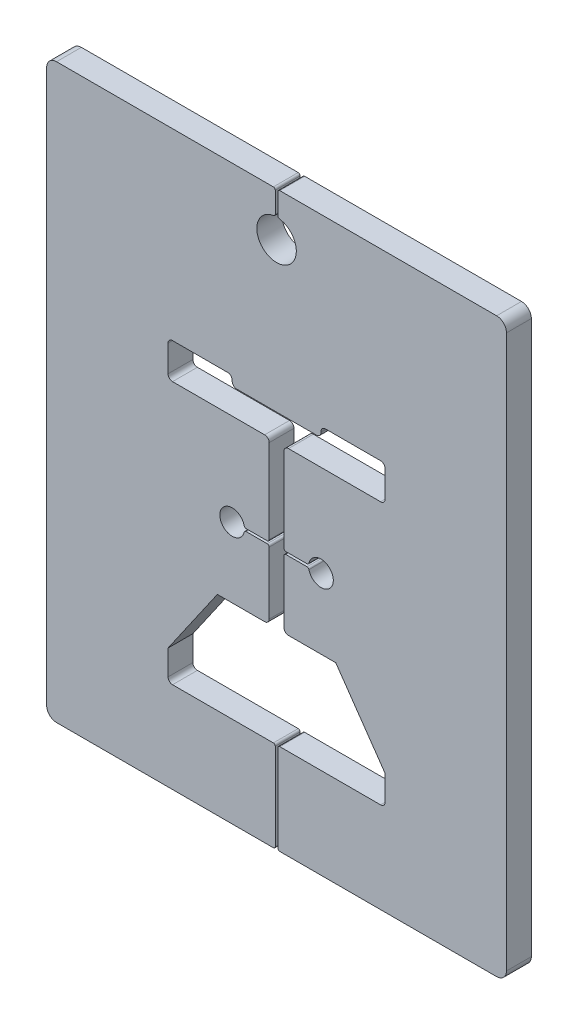
SolidWorks part; units mm, degrees
material "普通碳钢"
ref_plane "Front Plane" through (0, 0, 0) normal (0, 0, 1) x (1, 0, 0)
ref_plane "Top Plane" through (0, 0, 0) normal (0, 1, 0) x (1, 0, 0)
ref_plane "Right Plane" through (0, 0, 0) normal (1, 0, 0) x (0, 0, -1)
sketch "Sketch1" plane through (0, 0, 0) normal (0, 0, 1) x (1, 0, 0)
  line L0 (-190.5614, 818.5943) -> (-190.5614, -410.938) construction
  line L1 (-473.7714, 649.4855) -> (-194.7114, 649.4855)
  line L2 (-486.4714, 636.7855) -> (-486.4714, -74.4145)
  line L3 (-473.7714, -87.1145) -> (-194.7114, -87.1145)
  line L4 (105.3486, 636.7855) -> (105.3486, -74.4145)
  line L5 (-664.6272, 249.4355) -> (322.8712, 249.4355) construction
  line L6 (92.6486, 649.4855) -> (-186.4114, 649.4855)
  line L7 (-258.2687, 592.3355) -> (-244.68, 592.3355) construction
  line L8 (-192.2114, 646.9855) -> (-192.2114, 620.1833)
  line L9 (-188.9114, 646.9855) -> (-188.9114, 620.1833)
  line L10 (92.6486, -87.1145) -> (-186.4114, -87.1145)
  line L11 (-192.2114, -84.6145) -> (-192.2114, 27.2255)
  line L12 (-247.7114, 407.4655) -> (-247.7114, 406.3655)
  line L13 (-194.7114, 29.7255) -> (-324.4614, 29.7255)
  line L14 (-330.2614, 35.5255) -> (-330.2614, 67.7255)
  line L15 (-330.2614, 67.7255) -> (-266.7614, 159.2655)
  line L16 (-266.7614, 159.2655) -> (-205.8864, 159.2655)
  line L17 (-200.0864, 165.0655) -> (-200.0864, 245.2855)
  line L18 (-178.5364, 247.7855) -> (-151.3117, 247.7855)
  line L19 (-178.5364, 251.0855) -> (-151.3117, 251.0855)
  line L20 (-181.0364, 253.5855) -> (-181.0364, 302.7759)
  line L21 (-200.0864, 253.5855) -> (-200.0864, 302.7759)
  line L26 (-200.0864, 302.7759) -> (-200.0864, 361.7455)
  line L27 (-205.8864, 367.5455) -> (-324.4664, 367.5455)
  line L28 (-330.2664, 373.3455) -> (-330.2664, 407.4655)
  line L29 (-324.4664, 413.2655) -> (-253.5114, 413.2655)
  line L30 (-241.9114, 400.5655) -> (-139.2114, 400.5655)
  line L31 (-188.9114, -84.6145) -> (-188.9114, 27.2255)
  line L32 (-186.4114, 29.7255) -> (-56.6614, 29.7255)
  line L33 (-50.8614, 35.5255) -> (-50.8614, 67.7255)
  line L34 (-50.8614, 67.7255) -> (-114.3614, 159.2655)
  line L35 (-114.3614, 159.2655) -> (-175.2364, 159.2655)
  line L36 (-181.0364, 165.0655) -> (-181.0364, 245.2855)
  line L37 (-181.0364, 302.7759) -> (-181.0364, 361.7455)
  line L38 (-175.2364, 367.5455) -> (-56.6564, 367.5455)
  line L39 (-50.8564, 373.3455) -> (-50.8564, 407.4655)
  line L40 (-56.6564, 413.2655) -> (-127.6114, 413.2655)
  line L41 (-133.4114, 407.4655) -> (-133.4114, 406.3655)
  line L42 (-202.5864, 251.0855) -> (-229.8112, 251.0855)
  line L43 (-202.5864, 247.7855) -> (-229.8112, 247.7855)
  arc A0 (-194.3396, 617.7111) -> (-186.7833, 617.7111) centre (-190.5614, 592.5937) ccw
  arc A1 (-188.9114, 620.1833) -> (-186.7833, 617.7111) centre (-186.4114, 620.1833) ccw
  arc A2 (-192.2114, 620.1833) -> (-194.3396, 617.7111) centre (-194.7114, 620.1833) cw
  arc A3 (-188.9114, 646.9855) -> (-186.4114, 649.4855) centre (-186.4114, 646.9855) cw
  arc A4 (-192.2114, 646.9855) -> (-194.7114, 649.4855) centre (-194.7114, 646.9855) ccw
  arc A5 (-151.3117, 251.0855) -> (-148.8763, 253.0208) centre (-151.3117, 253.5855) ccw
  arc A6 (-148.8763, 245.8501) -> (-151.3117, 247.7855) centre (-151.3117, 245.2855) ccw
  arc A7 (-148.8763, 253.0208) -> (-148.8763, 245.8501) centre (-133.4114, 249.4355) cw
  arc A8 (-181.0364, 245.2855) -> (-178.5364, 247.7855) centre (-178.5364, 245.2855) cw
  arc A9 (-178.5364, 251.0855) -> (-181.0364, 253.5855) centre (-178.5364, 253.5855) cw
  arc A10 (-200.0864, 245.2855) -> (-202.5864, 247.7855) centre (-202.5864, 245.2855) ccw
  arc A11 (-200.0864, 253.5855) -> (-202.5864, 251.0855) centre (-202.5864, 253.5855) cw
  arc A15 (-188.9114, -84.6145) -> (-186.4114, -87.1145) centre (-186.4114, -84.6145) ccw
  arc A16 (-192.2114, -84.6145) -> (-194.7114, -87.1145) centre (-194.7114, -84.6145) cw
  arc A17 (-188.9114, 27.2255) -> (-186.4114, 29.7255) centre (-186.4114, 27.2255) cw
  arc A18 (-192.2114, 27.2255) -> (-194.7114, 29.7255) centre (-194.7114, 27.2255) ccw
  arc A19 (-486.4714, 636.7855) -> (-473.7714, 649.4855) centre (-473.7714, 636.7855) cw
  arc A20 (105.3486, 636.7855) -> (92.6486, 649.4855) centre (92.6486, 636.7855) ccw
  arc A21 (92.6486, -87.1145) -> (105.3486, -74.4145) centre (92.6486, -74.4145) ccw
  arc A22 (-486.4714, -74.4145) -> (-473.7714, -87.1145) centre (-473.7714, -74.4145) ccw
  arc A23 (-133.4114, 406.3655) -> (-139.2114, 400.5655) centre (-139.2114, 406.3655) cw
  arc A24 (-241.9114, 400.5655) -> (-247.7114, 406.3655) centre (-241.9114, 406.3655) cw
  arc A25 (-175.2364, 159.2655) -> (-181.0364, 165.0655) centre (-175.2364, 165.0655) cw
  arc A26 (-200.0864, 165.0655) -> (-205.8864, 159.2655) centre (-205.8864, 165.0655) cw
  arc A27 (-50.8614, 35.5255) -> (-56.6614, 29.7255) centre (-56.6614, 35.5255) cw
  arc A28 (-324.4614, 29.7255) -> (-330.2614, 35.5255) centre (-324.4614, 35.5255) cw
  arc A29 (-181.0364, 361.7455) -> (-175.2364, 367.5455) centre (-175.2364, 361.7455) cw
  arc A30 (-200.0864, 361.7455) -> (-205.8864, 367.5455) centre (-205.8864, 361.7455) ccw
  arc A31 (-133.4114, 407.4655) -> (-127.6114, 413.2655) centre (-127.6114, 407.4655) cw
  arc A32 (-247.7114, 407.4655) -> (-253.5114, 413.2655) centre (-253.5114, 407.4655) ccw
  arc A33 (-56.6564, 413.2655) -> (-50.8564, 407.4655) centre (-56.6564, 407.4655) cw
  arc A34 (-50.8564, 373.3455) -> (-56.6564, 367.5455) centre (-56.6564, 373.3455) cw
  arc A35 (-324.4664, 367.5455) -> (-330.2664, 373.3455) centre (-324.4664, 373.3455) cw
  arc A36 (-330.2664, 407.4655) -> (-324.4664, 413.2655) centre (-324.4664, 407.4655) cw
  arc A37 (-232.2466, 253.0208) -> (-232.2466, 245.8501) centre (-247.7114, 249.4355) ccw
  arc A38 (-232.2466, 245.8501) -> (-229.8112, 247.7855) centre (-229.8112, 245.2855) cw
  arc A39 (-229.8112, 251.0855) -> (-232.2466, 253.0208) centre (-229.8112, 253.5855) cw
  point P21 (-188.9114, 649.4855)
  point P24 (-192.2114, 649.4855)
  point P46 (-181.0364, 247.7855)
  point P49 (-181.0364, 251.0855)
  point P52 (-200.0864, 247.7855)
  point P56 (-200.0864, 251.0855)
  point P72 (-190.5614, 400.5655)
  point P86 (-188.9114, -87.1145)
  point P89 (-192.2114, -87.1145)
  point P92 (-188.9114, 29.7255)
  point P95 (-192.2114, 29.7255)
  point P98 (-486.4714, 649.4855)
  point P101 (105.3486, 649.4855)
  point P104 (105.3486, -87.1145)
  point P107 (-486.4714, -87.1145)
  point P110 (-133.4114, 400.5655)
  point P113 (-247.7114, 400.5655)
  point P116 (-181.0364, 159.2655)
  point P119 (-200.0864, 159.2655)
  point P122 (-50.8614, 29.7255)
  point P125 (-330.2614, 29.7255)
  point P128 (-181.0364, 367.5455)
  point P131 (-200.0864, 367.5455)
  point P134 (-133.4114, 413.2655)
  point P137 (-247.7114, 413.2655)
  point P140 (-50.8564, 413.2655)
  point P143 (-50.8564, 367.5455)
  point P146 (-330.2664, 367.5455)
  point P149 (-330.2664, 413.2655)
  dimension "D5" = 50.8
  dimension "D6" = 2.5
  dimension "D7" = 2.5
  dimension "D23" = 2.5
  dimension "D24" = 12.7
  dimension "D25" = 5.8
  dimension "D26" = 5.8
  dimension "D27" = 5.8
  dimension "D28" = 5.8
  dimension "D32" = 31.75
  dimension "D33" = 2.5
  dimension "D16" = 2.5
  dimension "D1" = 736.6
  dimension "D2" = 591.82
  dimension "D3" = 3.3
  dimension "D4" = 57.15
  dimension "D8" = 3.3
  dimension "D9" = 116.84
  dimension "D10" = 139.705
  dimension "D11" = 138.05
  dimension "D12" = 38
  dimension "D13" = 76.2
  dimension "D14" = 9.525
  dimension "D15" = 208.28
  dimension "D17" = 236.22
  dimension "D20" = 57.15
  dimension "D22" = 45.72
  dimension "D29" = 12.7
  dimension "D30" = 400.05
  dimension "D31" = 3.3
extrude "Boss-Extrude1" add sketch "Sketch1" along normal blind 32
